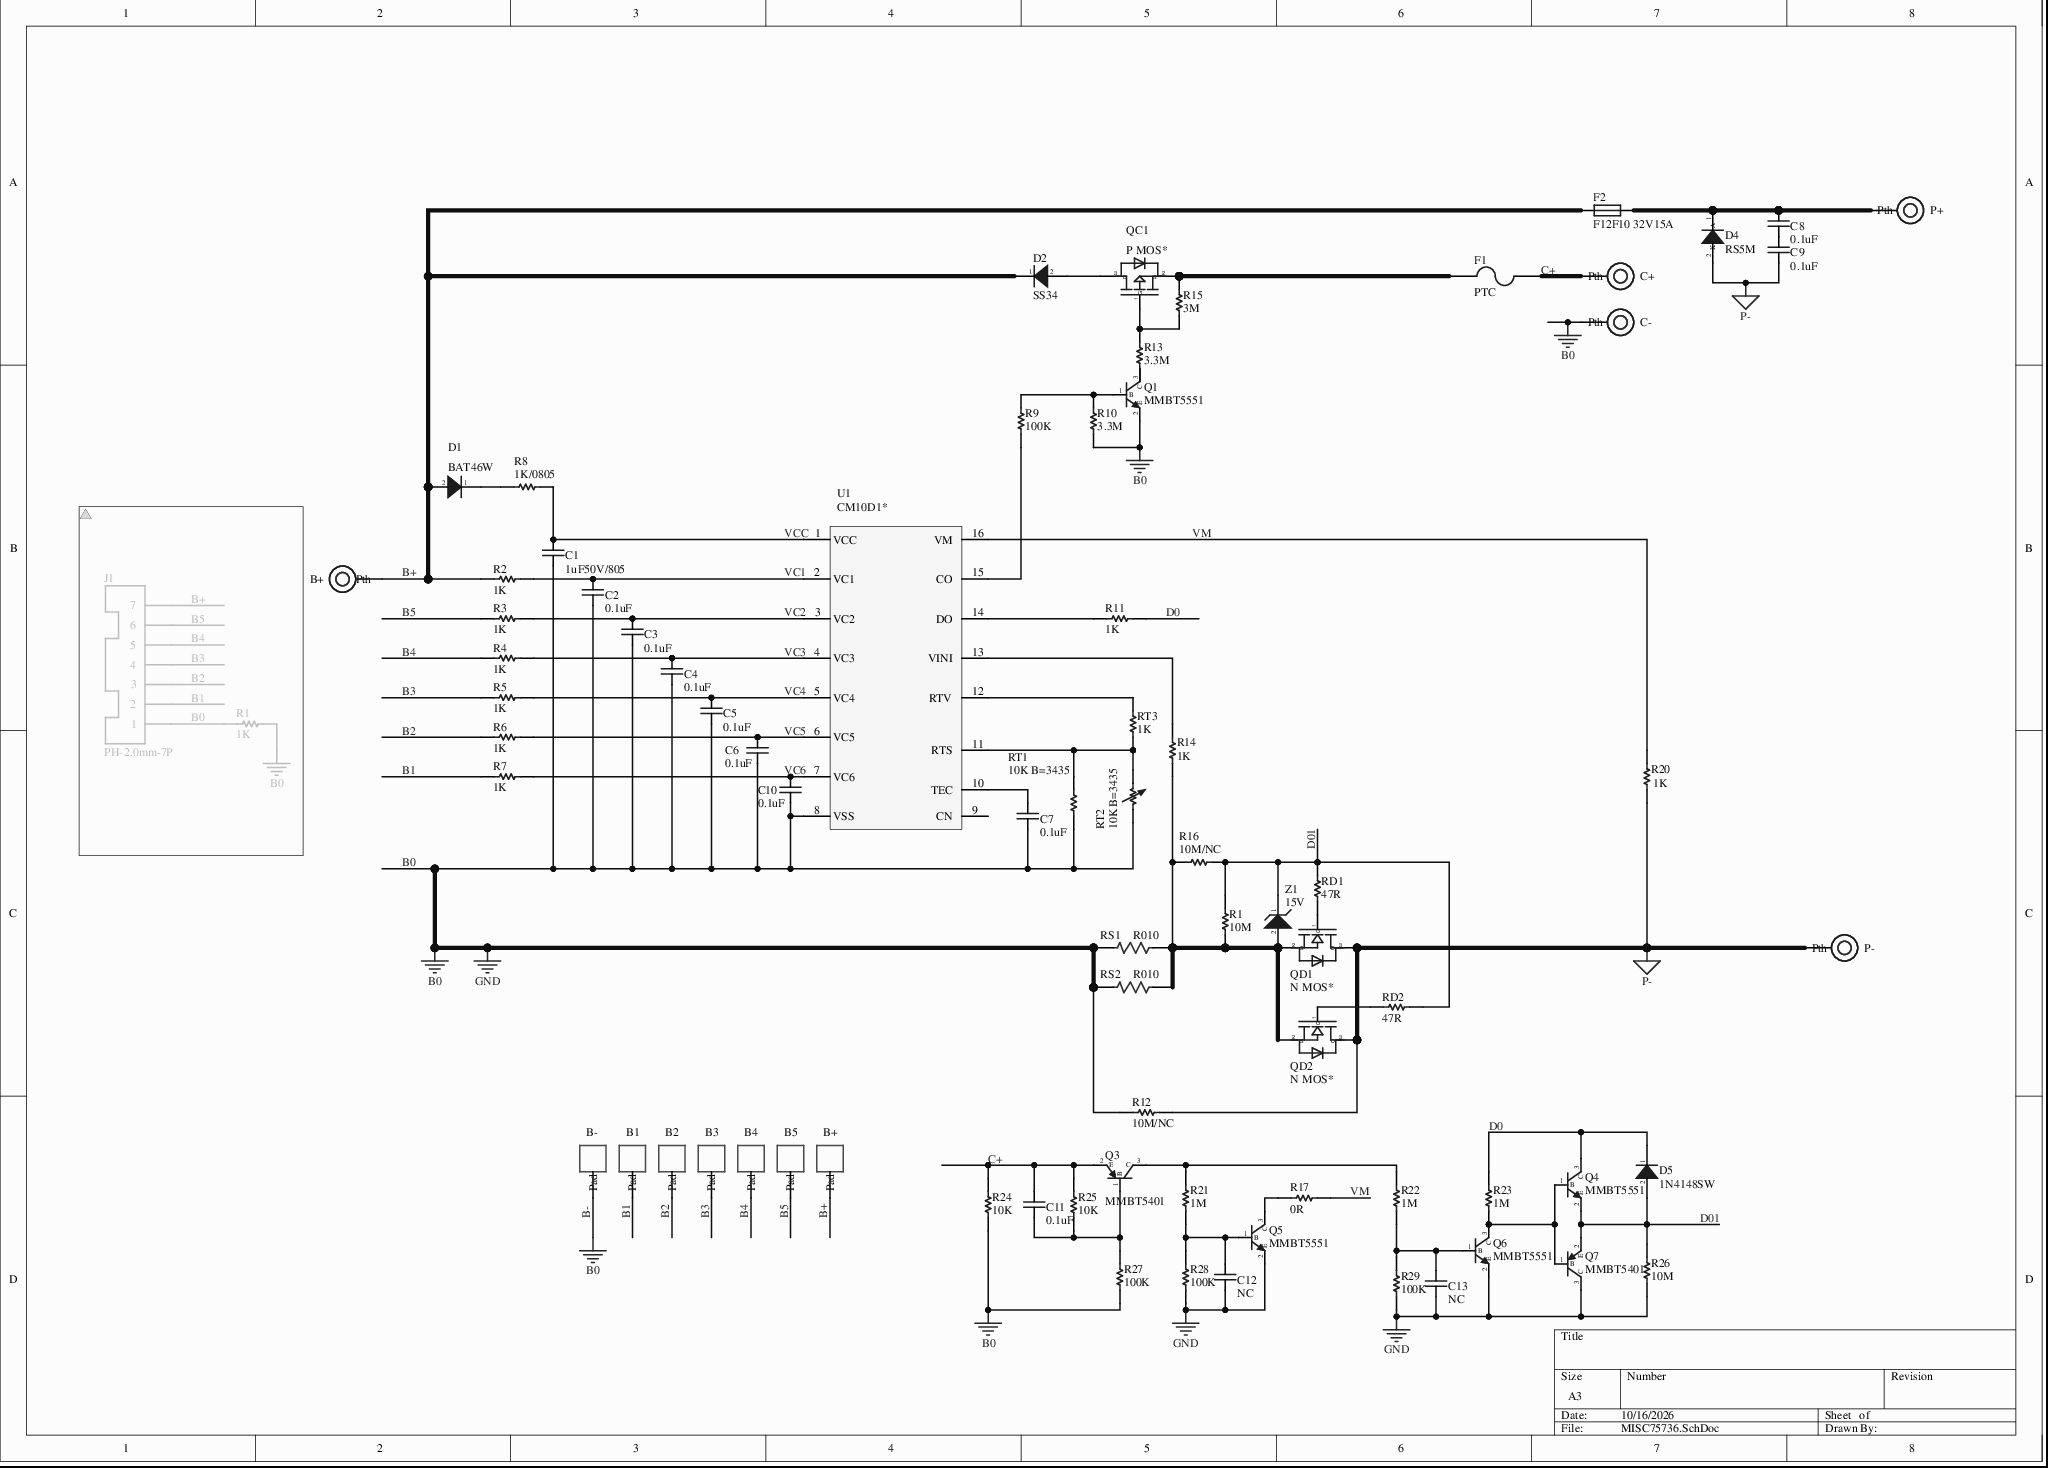
[diagram p0: MISC75736.SchDoc]
# Altium project MISC75736.PrjPcb
1 sheet, 78 parts. Net scope: global (net labels, ports and power ports of the same name join across sheets).
Board file: MISC75736.PcbDoc

## Sheet MISC75736.SchDoc
size A3; SheetNumber: 1; SheetTotal: 1

### Parts
(Parts that share a designator on the sheet are numbered #1, #2 ... from top to bottom, then left to right.)
B1  Pad  [Pad10X8mm]
B2  Pad  [Pad10X8mm]
B3  Pad  [Pad10X8mm]
B4  Pad  [Pad10X8mm]
B5  Pad  [Pad10X8mm]
B+#1  Pth  [4*3]
B+#2  Pad  [Pad10X8mm]
B-  Pad  [Pad10X8mm]
C1  1uF50V/805  [C0805L]
C2  0.1uF  [C0603A]
C3  0.1uF  [C0603A]
C4  0.1uF  [C0603A]
C5  0.1uF  [C0603A]
C6  0.1uF  [C0603A]
C7  0.1uF  [C0603A]
C8  0.1uF  [C0603A]
C9  0.1uF  [C0603A]
C10  0.1uF  [C0603A]
C11  0.1uF  [C0603A]
C12  NC  [C0603A]
C13  NC  [C0603A]
C+  Pth  [4*3]
C-  Pth  [4*3]
D1  BAT46W  [SOD323]
D2  SS34  [SMB(DO-214AA)]
D4  RS5M  [SMC A(DO-214AB)]
D5  1N4148SW  [SOD323]
F1  PTC  [F1812A]
F2  F12F10 32V15A  [R1206A]
J1  PH-2.0mm-7P  (masked out: inside a compile mask, not in the netlist)
P+  Pth  [4*3]
P-  Pth  [4*3]
Q1  MMBT5551  [SOT23-3]
Q3  MMBT5401  [SOT23-3]
Q4  MMBT5551  [SOT23-3]
Q5  MMBT5551  [SOT23-3]
Q6  MMBT5551  [SOT23-3]
Q7  MMBT5401  [SOT23-3]
QC1  P MOS*  [SOP-8L(T3p)]
QD1  N MOS*  [TO-252]
QD2  N MOS*  [TO-252]
R1#1  1K  [R0805L]  (masked out: inside a compile mask, not in the netlist)
R1#2  10M  [R0603A]
R2  1K  [R0603A]
R3  1K  [R0603A]
R4  1K  [R0603A]
R5  1K  [R0603A]
R6  1K  [R0603A]
R7  1K  [R0603A]
R8  1K/0805  [R0805L]
R9  100K  [R0603A]
R10  3.3M  [R0603A]
R11  1K  [R0603A]
R12  10M/NC  [R0603A]
R13  3.3M  [R0603A]
R14  1K  [R0603A]
R15  3M  [R0603A]
R16  10M/NC  [R0603A]
R17  0R  [R0603A]
R20  1K  [R0603A]
R21  1M  [R0603A]
R22  1M  [R0603A]
R23  1M  [R0603A]
R24  10K  [R0603A]
R25  10K  [R0603A]
R26  10M  [R0603A]
R27  100K  [R0603A]
R28  100K  [R0603A]
R29  100K  [R0603A]
RD1  47R  [R0603A]
RD2  47R  [R0603A]
RS1  R010  [R2512L]
RS2  R010  [R2512L]
RT1  10K B=3435  [R0603A]
RT2  10K B=3435  [R0603A]
RT3  1K  [R0603A]
U1  CM10D1*  [SOP16L]
Z1  15V  [SOD323]

### Nets
B0: B-.1 C1.1 C2.1 C3.1 C4.1 C5.1 C6.1 C7.2 C10.1 C12.2 C13.2 C-.1 Q1.2(E) Q5.2(E) Q6.2(E) Q7.3(C) R10.1 R12.1 R24.1 R26.1 R27.1 R28.1 R29.1 RS1.1 RS2.1 RT1.1 RT2.1 U1.8(VSS)  [also labelled B-, GND]
P-: C9.2 D4.2(K) P-.1 QD1.3(D) QD2.3(D) R12.2 R20.1
B1: B1.1 R7.1
B2: B2.1 R6.1
B3: B3.1 R5.1
B4: B4.1 R4.1
B5: B5.1 R3.1
B+: B+#1.1 B+#2.1 D1.2(K) D2.1(A) F2.1 R2.1
C+: C11.1 C+.1 F1.2 Q3.2(E) R24.2 R25.2
D0: D5.1(A) Q4.3(C) R11.1 R23.2
D01: D5.2 Q4.2(E) Q7.2(E) R1#2.2 R16.2 R26.2 RD1.1 RD2.2 Z1.1(A)
VC1: C2.2 R2.2 U1.2(VC1)
VC2: C3.2 R3.2 U1.3(VC2)
VC3: C4.2 R4.2 U1.4(VC3)
VC4: C5.2 R5.2 U1.5(VC4)
VC5: C6.2 R6.2 U1.6(VC5)
VC6: C10.2 R7.2 U1.7(VC6)
VCC: C1.2 R8.2 U1.1(VCC)
VM: R17.1 R20.2 U1.16(VM)
NetC7_1: C7.1 U1.10(TEC)
NetC8_1: C8.1 D4.1(A) F2.2 P+.1
NetC8_2: C8.2 C9.1
NetC11_2: C11.2 Q3.1(B) R25.1 R27.2
NetC12_1: C12.1 Q5.1(B) R21.1 R28.2
NetC13_1: C13.1 Q6.1(B) R22.1 R29.2
NetD1_1: D1.1(A) R8.1
NetD2_2: D2.2(K) QC1.3(D)
NetF1_1: F1.1 QC1.2(S) R15.2
NetQ1_1: Q1.1(B) R9.2 R10.2
NetQ1_3: Q1.3(C) R13.1
NetQ3_3: Q3.3(C) R21.2 R22.2
NetQ4_1: Q4.1(B) Q6.3(C) Q7.1(B) R23.1
NetQ5_3: Q5.3(C) R17.2
NetQC1_1: QC1.1(G) R13.2 R15.1
NetQD1_1: QD1.1(G) RD1.2
NetQD1_2: QD1.2(S) QD2.2(S) R1#2.1 R14.1 R16.1 RS1.2 RS2.2 Z1.2(K)
NetQD2_1: QD2.1(G) RD2.1
NetR9_1: R9.1 U1.15(CO)
NetR11_2: R11.2 U1.14(DO)
NetR14_2: R14.2 U1.13(VINI)
NetRT1_2: RT1.2 RT2.2 RT3.1 U1.11(RTS)
NetRT3_2: RT3.2 U1.12(RTV)

Not connected (* = marked no-connect by the designer): U1 9(CN)*

### Library data of the parts
B1-B5 B+#2 B- = Pad: connection pad (non-through-hole)
B+#1 C+ C- P+ P- = Pth: through-hole pad
C1-C13 = CAP: chip capacitor
D1 = BAT46W: chip diode
D2 = SS34: chip Schottky diode
D4 = RS5M: chip diode
D5 = 1N4148SW: chip diode
F1 = PTC: chip resettable fuse
F2 = FUSE
J1 = PH-2.0mm-7P: connector
Q1 Q4-Q6 = MMBT5551: chip transistor
Q3 Q7 = MMBT5401: chip transistor
QC1 = P MOS*: chip MOSFET
QD1 QD2 = N MOS*: chip MOSFET
R1#1 R1#2 R2-R17 R20-R29 RD1 RD2 RT1 RT3 = RES: chip resistor
RS1 RS2 = RES2: chip metal alloy resistor
RT2 = NTC: chip thermistor
U1 = CM1061*: 6-cell battery protection IC
Z1 = 15V: chip Zener diode